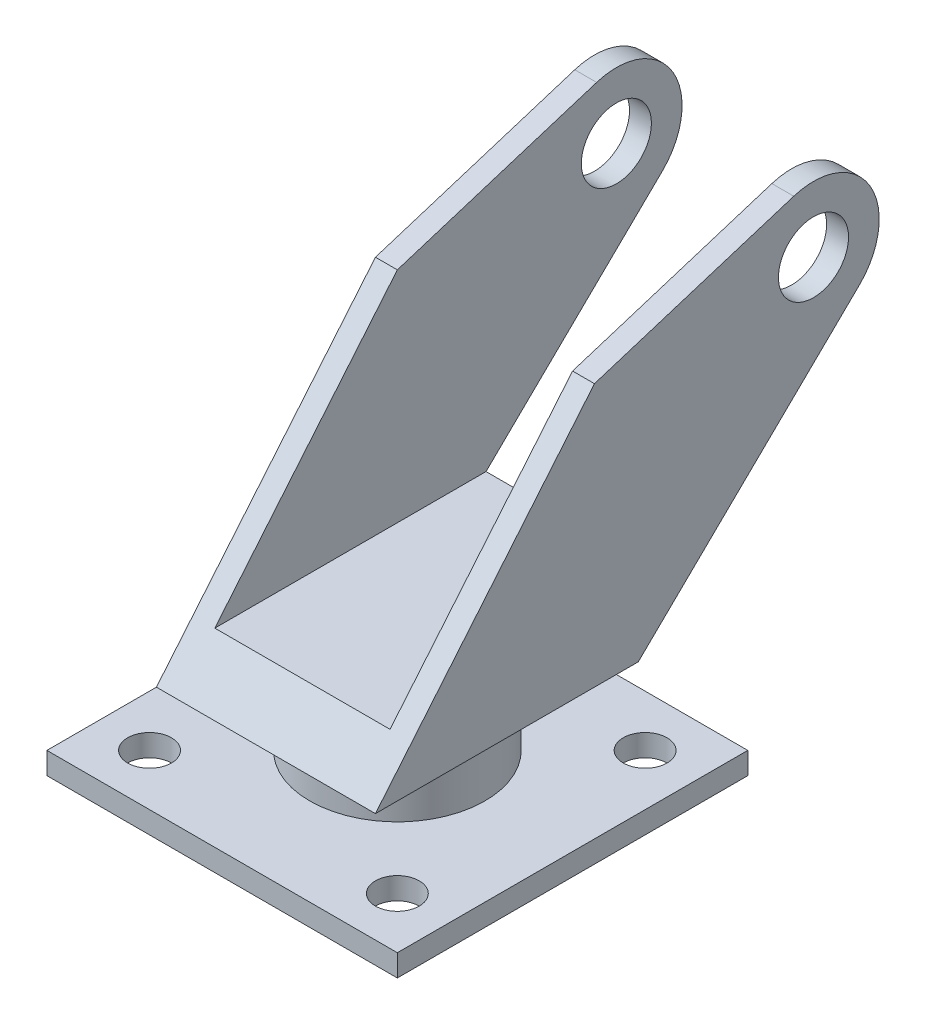
SolidWorks part; units mm, degrees
ref_plane "Front Plane" through (0, 0, 0) normal (0, 0, 1) x (1, 0, 0)
ref_plane "Top Plane" through (0, 0, 0) normal (0, 1, 0) x (1, 0, 0)
ref_plane "Right Plane" through (0, 0, 0) normal (1, 0, 0) x (0, 0, -1)
other "Configuration Table"
sketch "Sketch1" plane through (0, 0, 0) normal (0, 1, 0) x (1, 0, 0)
  line L1 (-40, 40) -> (40, 40)
  line L2 (-40, 40) -> (-40, -40)
  line L3 (-40, -40) -> (40, -40)
  line L4 (40, 40) -> (40, -40)
  line L5 (-40, 40) -> (40, -40) construction
  line L6 (-40, -40) -> (40, 40) construction
  circle A0 centre (-28.2843, -28.2843) radius 5
  circle A1 centre (-28.2843, 28.2843) radius 5
  circle A2 centre (28.2843, 28.2843) radius 5
  circle A3 centre (28.2843, -28.2843) radius 5
  point P0 (0, 0)
  point P17 (0, 0)
  dimension "D4" = 10
  dimension "D1" = 80
  dimension "D2" = 80
  dimension "D3" = 4
extrude "Boss-Extrude3" add sketch "Sketch1" along normal blind 5
sketch "Sketch3" plane through (0, 5, 0) normal (0, 1, 0) x (1, 0, 0)
  circle A0 centre (0, 0) radius 20
  dimension "D1" = 40
extrude "Boss-Extrude4" add sketch "Sketch3" along normal blind 15
sketch "Sketch6" plane through (0, 0, 0) normal (1, 0, 0) x (0, 0, -1)
  line L1 (20, 20) -> (-20, 20) construction
  line L2 (0, 20) -> (30, 20)
  line L7 (30, 20) -> (80.477, 69.2653)
  line L8 (20, 80) -> (65.5, 94.3091)
  line L9 (0, 20) -> (-30, 20)
  line L10 (-30, 20) -> (20, 80)
  arc A0 (80.477, 69.2653) -> (65.5, 94.3091) centre (70, 80) ccw
  circle A1 centre (70, 80) radius 8
  dimension "D4" = 30
  dimension "D2" = 16
  dimension "D1" = 30
  dimension "D3" = 50
  dimension "D5" = 30
ref_plane "Plane2" through (0, 80, 0) normal (0, -1, 0) x (-1, 0, 0)
sketch "Sketch8" plane through (0, 80, 0) normal (0, -1, 0) x (-1, 0, 0)
  line L1 (-20, 100) -> (20, 100)
  line L2 (-20, 100) -> (-20, -100)
  line L3 (-20, -100) -> (20, -100)
  line L4 (20, 100) -> (20, -100)
  line L5 (-20, 100) -> (20, -100) construction
  line L6 (-20, -100) -> (20, 100) construction
  point P1 (0, 0)
  dimension "D1" = 200
  dimension "D2" = 40
extrude "Boss-Extrude6" add sketch "Sketch6" along normal blind 25 and the other way blind 25
extrude "Cut-Extrude1" cut sketch "Sketch8" against normal blind 25 and the other way blind 50
sketch "Sketch9" plane through (25, 0, 0) normal (1, 0, 0) x (0, 0, -1)
